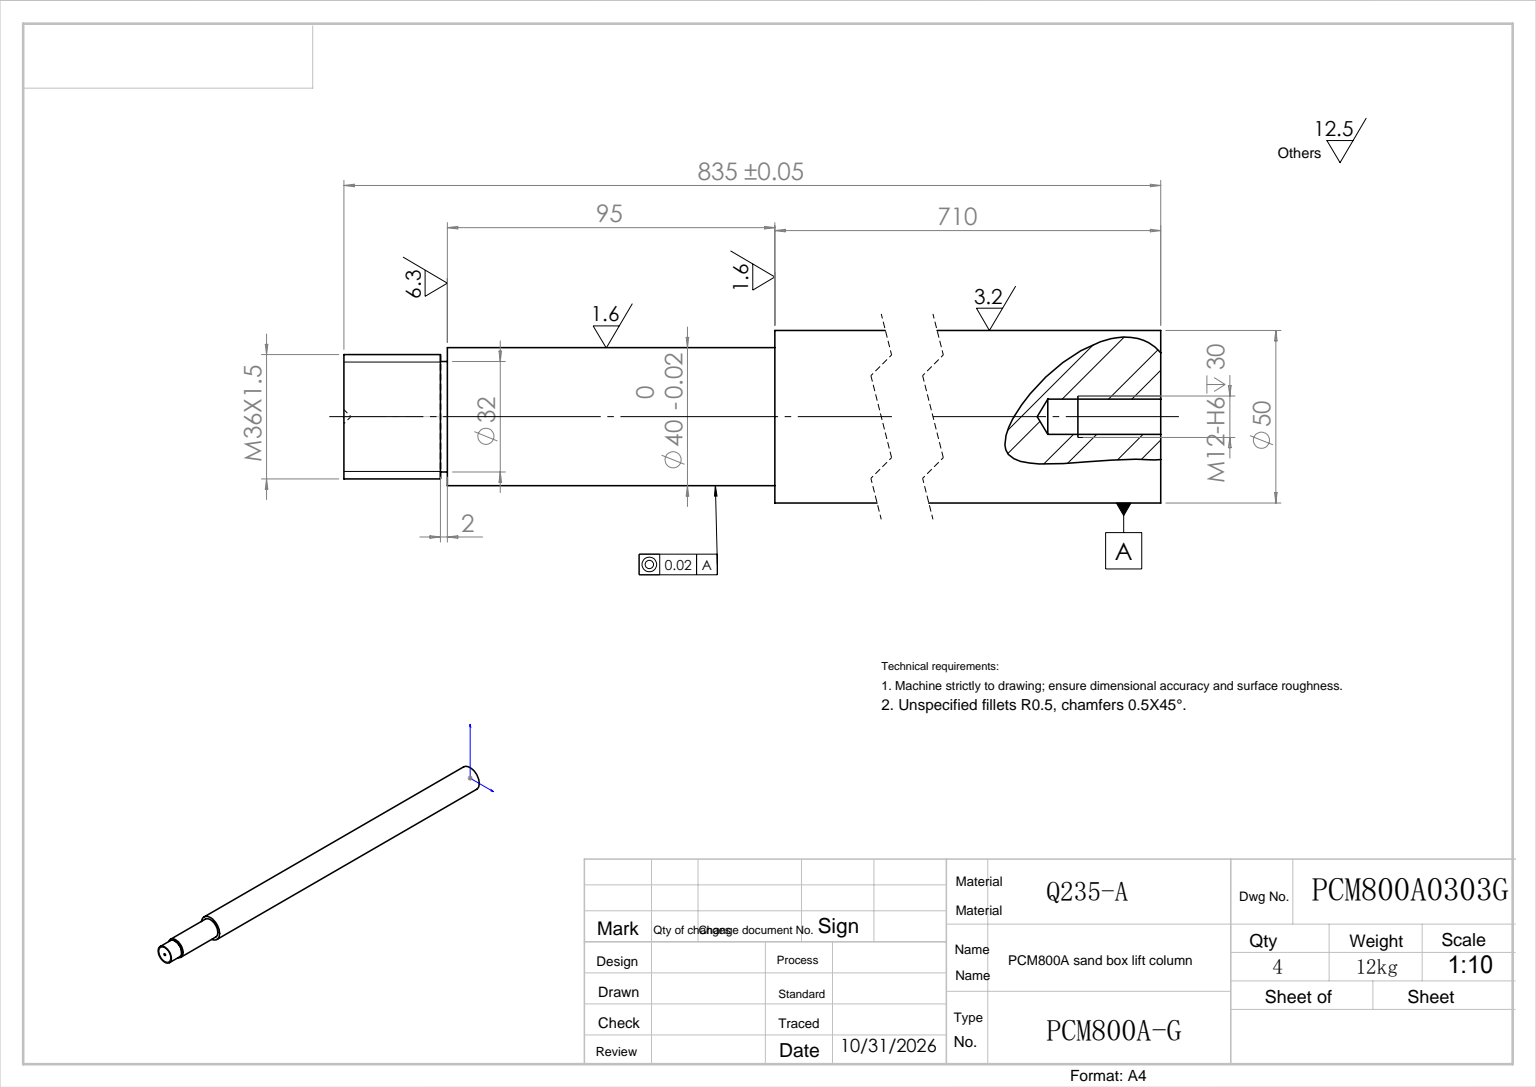
from build123d import *

# Parameters (mm, degrees)
SKETCH_1_R              = 25
EXTRUDE_1_DEPTH         = 710
SKETCH_2_R              = 20
EXTRUDE_2_DEPTH         = 95
SKETCH_3_R              = 18
EXTRUDE_3_DEPTH         = 30
HOLE_WIZARD_M12_1_D     = 10.2
HOLE_WIZARD_M12_1_DEPTH = 32.75
HOLE_WIZARD_M12_1_TIP   = 3.064389157
SKETCH_8_R              = 20
SKETCH_8_R_2            = 16
CUT_EXTRUDE_1_DEPTH     = 2


with BuildPart() as part:
    # 草图1 → 拉伸1 (new body)
    with BuildSketch(Plane.XY):
        Circle(SKETCH_1_R)
    extrude(amount=EXTRUDE_1_DEPTH)

    # 草图2 → 拉伸2 (add)
    with BuildSketch(Plane.XY.offset(710)):
        Circle(SKETCH_2_R)
    extrude(amount=EXTRUDE_2_DEPTH)

    # 草图3 → 拉伸3 (add)
    with BuildSketch(Plane.XY.offset(805)):
        Circle(SKETCH_3_R)
    extrude(amount=EXTRUDE_3_DEPTH)

    # M12 螺纹孔1
    with Locations(Plane(origin=(0, 0, 0), x_dir=(-1, 0, 0), z_dir=(0, 0, -1))):
        with Locations((0, 0)):
            Hole(HOLE_WIZARD_M12_1_D / 2, depth=HOLE_WIZARD_M12_1_DEPTH)
            with Locations((0, 0, -(HOLE_WIZARD_M12_1_DEPTH + HOLE_WIZARD_M12_1_TIP / 2))):  # 118° drill point
                Cone(0, HOLE_WIZARD_M12_1_D / 2, HOLE_WIZARD_M12_1_TIP, mode=Mode.SUBTRACT)

    # 草图7 → 切除-旋转1 (revolve, cut)
    with BuildSketch(Plane(origin=(0, 0, 0), x_dir=(1, 0, 0), z_dir=(0, 1, 0))):
        Polygon((-2, -835), (0, -833), (0, -835), align=None)
    revolve(axis=Axis((0, 0, 835), (0, 0, -1)), mode=Mode.SUBTRACT)

    # 草图8 → 切除-拉伸1 (cut)
    with BuildSketch(Plane.XY.offset(805)):
        Circle(SKETCH_8_R)
        Circle(SKETCH_8_R_2, mode=Mode.SUBTRACT)
    extrude(amount=CUT_EXTRUDE_1_DEPTH, mode=Mode.SUBTRACT)


solid = part.part
